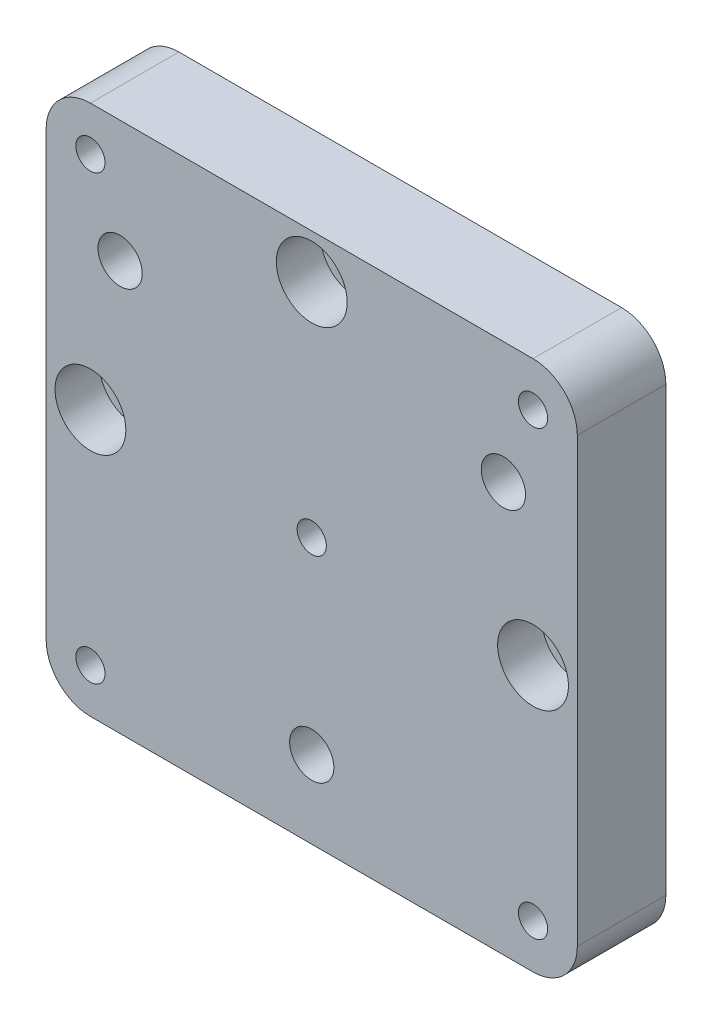
from build123d import *

# Parameters (mm, degrees)
SKETCH1_W             = 60
SKETCH1_H             = 60
BOSS_EXTRUDE1_DEPTH   = 10
FILLET1_R             = 5
M6_TAPPED_HOLE1_D     = 5
M6_TAPPED_HOLE1_DEPTH = 15
M6_TAPPED_HOLE1_TIP   = 1.502151548
SKETCH8_R             = 2.1
CUT_EXTRUDE1_DEPTH    = 51.336896077
SKETCH9_R             = 4
CUT_EXTRUDE2_DEPTH    = 5
M4_TAPPED_HOLE1_D     = 3.3
M4_TAPPED_HOLE2_D     = 3.3


with BuildPart() as part:
    # Sketch1 → Boss-Extrude1 (new body)
    with BuildSketch(Plane.XY):
        with Locations((9.163798419, 0)):
            Rectangle(SKETCH1_W, SKETCH1_H)
    extrude(amount=BOSS_EXTRUDE1_DEPTH)

    # Fillet1
    fillet1_edges = [part.edges().sort_by_distance(p)[0] for p in [
        (-20.836201581, 30, 5),
        (39.163798419, 30, 5),
        (39.163798419, -30, 5),
        (-20.836201581, -30, 5),
    ]]
    fillet(fillet1_edges, radius=FILLET1_R)

    # M6 Tapped Hole1
    with Locations(Plane.XY.offset(10)):
        with Locations((9.163798419, -21.25), (30.814433514, 16.25), (-12.486836675, 16.25)):
            Hole(M6_TAPPED_HOLE1_D / 2, depth=M6_TAPPED_HOLE1_DEPTH)
            with Locations((0, 0, -(M6_TAPPED_HOLE1_DEPTH + M6_TAPPED_HOLE1_TIP / 2))):  # 118° drill point
                Cone(0, M6_TAPPED_HOLE1_D / 2, M6_TAPPED_HOLE1_TIP, mode=Mode.SUBTRACT)

    # Sketch8 → Cut-Extrude1 (cut, through all)
    with BuildSketch(Plane.XY.offset(10)):
        with Locations((9.163798419, 25)):
            Circle(SKETCH8_R)
        with Locations((34.163798419, 0)):
            Circle(SKETCH8_R)
        with Locations((-15.836201581, 0)):
            Circle(SKETCH8_R)
    extrude(amount=-CUT_EXTRUDE1_DEPTH, mode=Mode.SUBTRACT)

    # Sketch9 → Cut-Extrude2 (cut)
    with BuildSketch(Plane.XY.offset(10)):
        with Locations((-15.836201581, 0)):
            Circle(SKETCH9_R)
        with Locations((9.163798419, 25)):
            Circle(SKETCH9_R)
        with Locations((34.163798419, 0)):
            Circle(SKETCH9_R)
    extrude(amount=-CUT_EXTRUDE2_DEPTH, mode=Mode.SUBTRACT)

    # M4 Tapped Hole1 (through all)
    with Locations(Plane.XY.offset(10)):
        with Locations((-15.836201581, -25), (34.163798419, -25), (34.163798419, 25), (-15.836201581, 25)):
            Hole(M4_TAPPED_HOLE1_D / 2)

    # M4 Tapped Hole2 (through all)
    with Locations(Plane.XY.offset(10)):
        with Locations((9.163798419, 0)):
            Hole(M4_TAPPED_HOLE2_D / 2)


solid = part.part
